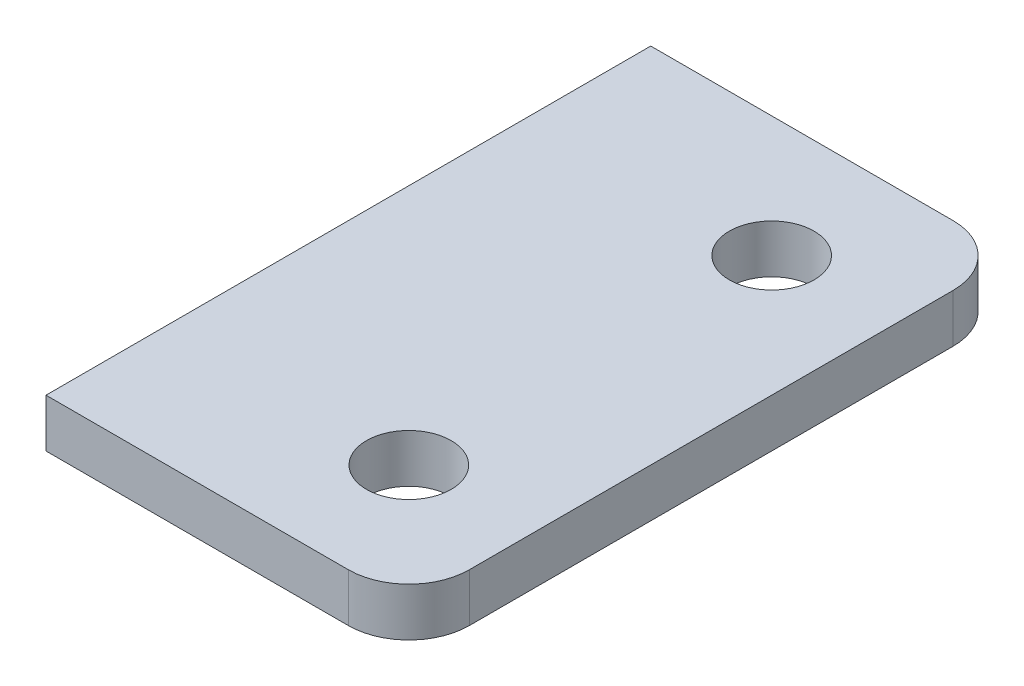
from build123d import *

# Parameters (mm, degrees)
SKETCH1_R           = 7
BOSS_EXTRUDE1_DEPTH = 8


with BuildPart() as part:
    # Sketch1 → Boss-Extrude1 (new body)
    with BuildSketch(Plane(origin=(0, 0, 0), x_dir=(1, 0, 0), z_dir=(0, 1, 0))):
        with BuildLine():
            Line((-30, -50), (20, -50))
            ThreePointArc((20, -50), (27.071067812, -47.071067812), (30, -40))
            Line((30, -40), (30, 40))
            ThreePointArc((30, 40), (27.071067812, 47.071067812), (20, 50))
            Line((20, 50), (-30, 50))
            Line((-30, 50), (-30, -50))
        make_face()
        with Locations(Location((10, 30, 0), (0, 0, 270))):
            Circle(SKETCH1_R, mode=Mode.SUBTRACT)
        with Locations(Location((10, -30, 0), (0, 0, 90))):
            Circle(SKETCH1_R, mode=Mode.SUBTRACT)
    extrude(amount=BOSS_EXTRUDE1_DEPTH)


solid = part.part
